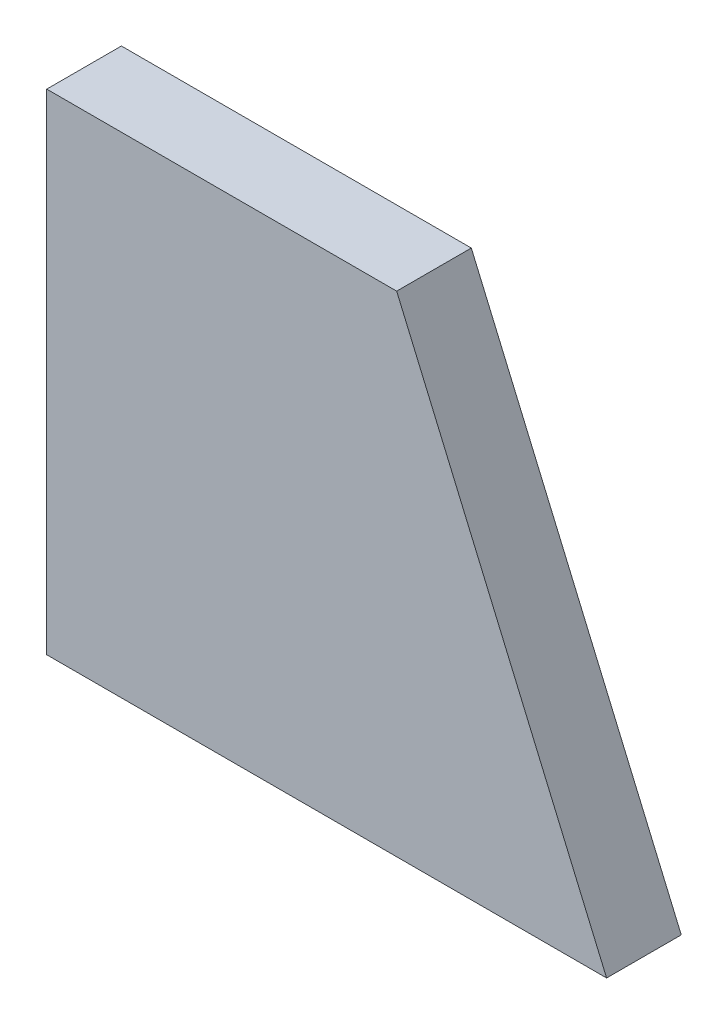
from build123d import *

# Parameters (mm, degrees)
BOSS_EXTRUDE1_DEPTH = 8


with BuildPart() as part:
    # Sketch1 → Boss-Extrude1 (new, symmetric)
    with BuildSketch(Plane.XY):
        Polygon((0, 0), (0, 105), (75, 105), (120, 0), align=None)
    extrude(amount=BOSS_EXTRUDE1_DEPTH, both=True)


solid = part.part
